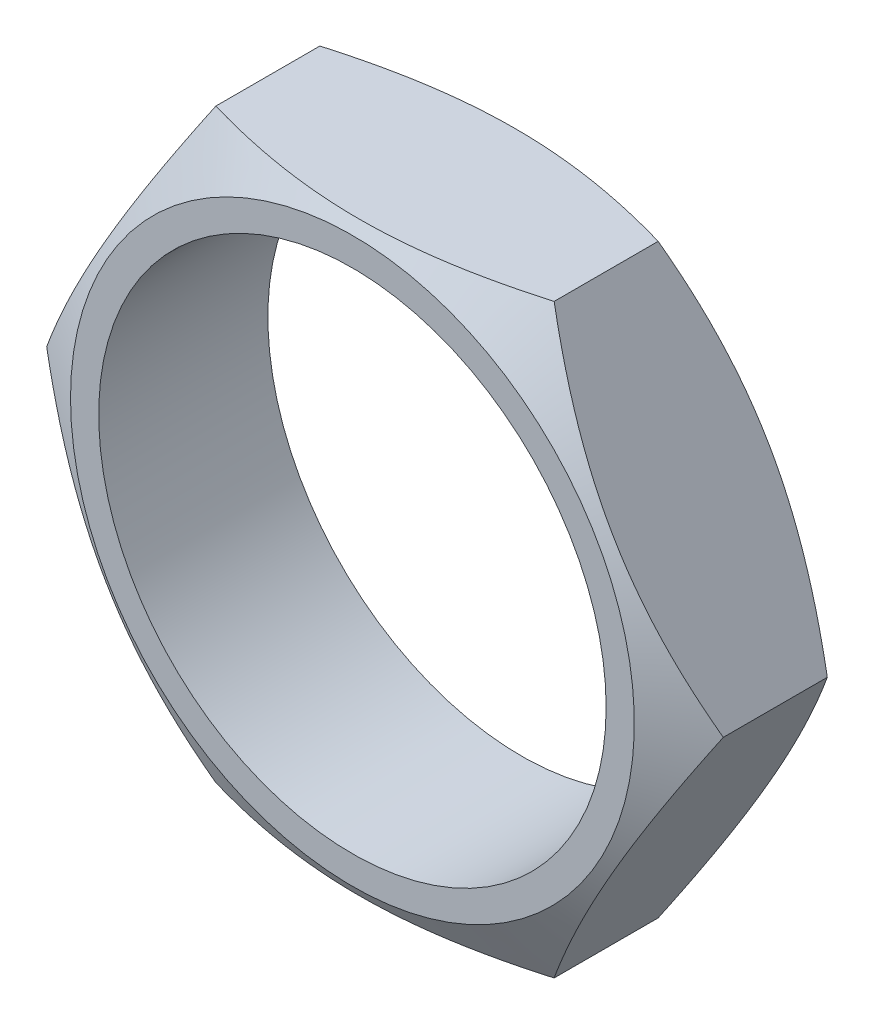
from build123d import *

# Parameters (mm, degrees)
SKETCH_1_R      = 18
EXTRUDE_1_DEPTH = 12


with BuildPart() as part:
    # 草图1 → 凸台-拉伸1 (new body)
    with BuildSketch(Plane.XY):
        Polygon((24, 0), (12, 20.784609691), (-12, 20.784609691), (-24, 0), (-12, -20.784609691), (12, -20.784609691), align=None)
        Circle(SKETCH_1_R, mode=Mode.SUBTRACT)
    extrude(amount=EXTRUDE_1_DEPTH)

    # 草图2 → 切除-旋转1 (revolve, cut)
    with BuildSketch(Plane(origin=(0, 0, 0), x_dir=(1, 0, 0), z_dir=(0, 1, 0))):
        Polygon((-24, 0), (-24, -2.309401077), (-20, 0), align=None)
        Polygon((-24, -12), (-24, -9.690598923), (-20, -12), align=None)
    revolve(axis=Axis((0, 0, -5.971832554), (0, 0, 1)), mode=Mode.SUBTRACT)


solid = part.part
